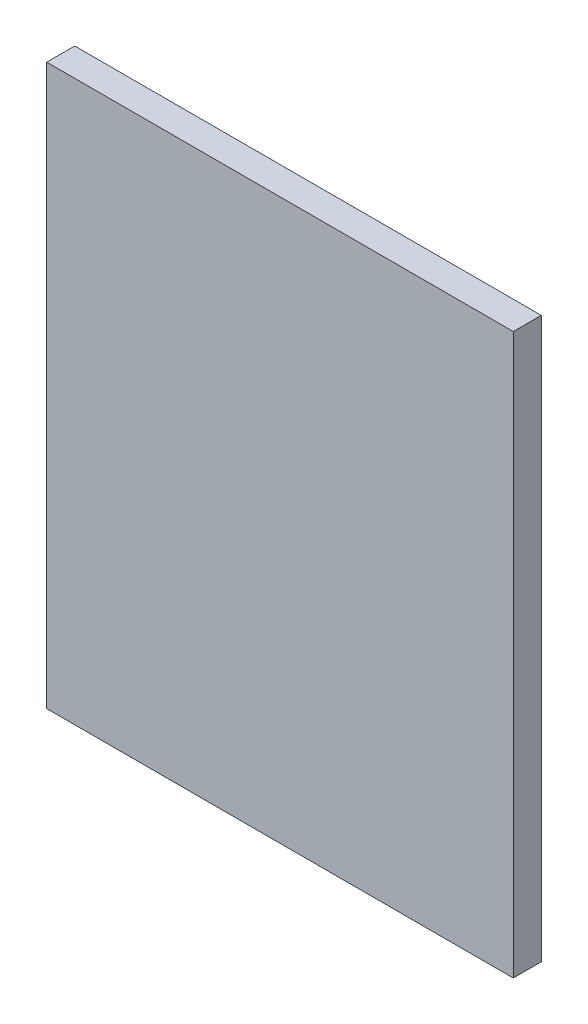
from build123d import *

# Parameters (mm, degrees)
SKETCH_1_W      = 100
SKETCH_1_H      = 120
EXTRUDE_1_DEPTH = 6


with BuildPart() as part:
    # 草图1 → 凸台-拉伸1 (new body)
    with BuildSketch(Plane.XY):
        with Locations((50, 60)):
            Rectangle(SKETCH_1_W, SKETCH_1_H)
    extrude(amount=EXTRUDE_1_DEPTH)


solid = part.part
